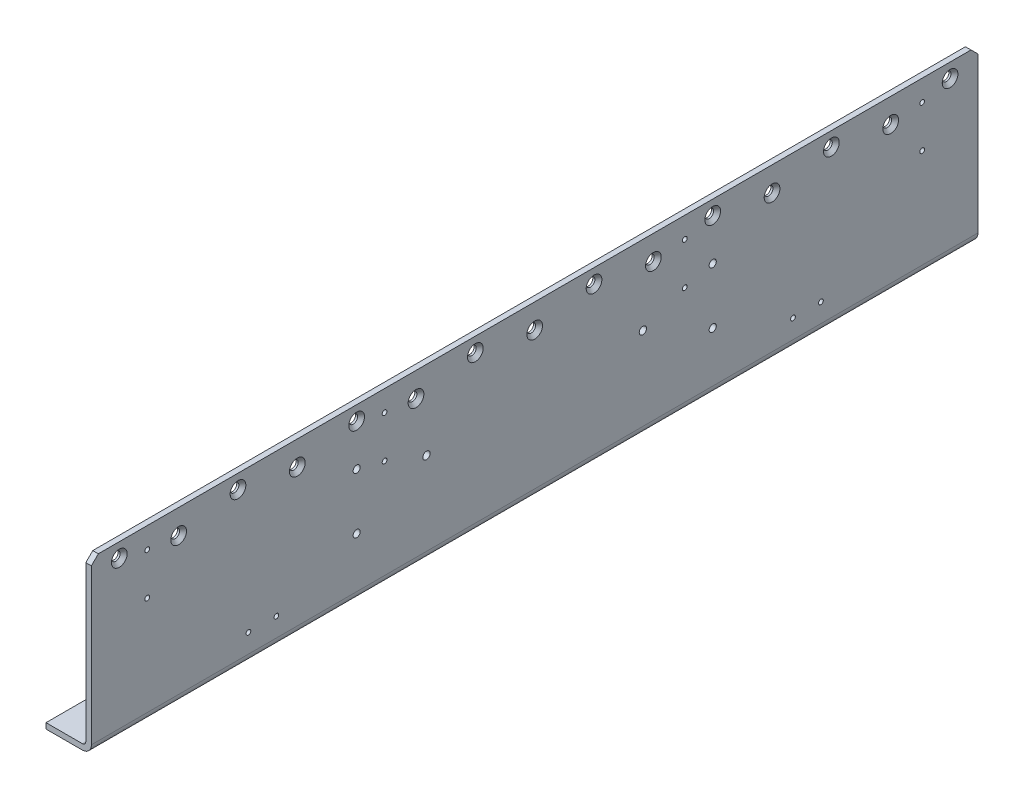
from build123d import *

# Parameters (mm, degrees)
BOSS_EXTRUDE1_DEPTH           = 1270
SKETCH3_R                     = 6.25
CUT_EXTRUDE1_DEPTH            = 3
SKETCH4_R                     = 6.25
CUT_EXTRUDE2_DEPTH            = 5
CUT_EXTRUDE2_DRAFT            = 45
CUT_EXTRUDE2_PROFILE_2_DEPTH  = 5
CUT_EXTRUDE2_PROFILE_2_DRAFT  = 45
CUT_EXTRUDE2_PROFILE_3_DEPTH  = 5
CUT_EXTRUDE2_PROFILE_3_DRAFT  = 45
CUT_EXTRUDE2_PROFILE_4_DEPTH  = 5
CUT_EXTRUDE2_PROFILE_4_DRAFT  = 45
CUT_EXTRUDE2_PROFILE_5_DEPTH  = 5
CUT_EXTRUDE2_PROFILE_5_DRAFT  = 45
CUT_EXTRUDE2_PROFILE_6_DEPTH  = 5
CUT_EXTRUDE2_PROFILE_6_DRAFT  = 45
CUT_EXTRUDE2_PROFILE_7_DEPTH  = 5
CUT_EXTRUDE2_PROFILE_7_DRAFT  = 45
CUT_EXTRUDE2_PROFILE_8_DEPTH  = 5
CUT_EXTRUDE2_PROFILE_8_DRAFT  = 45
CUT_EXTRUDE2_PROFILE_9_DEPTH  = 5
CUT_EXTRUDE2_PROFILE_9_DRAFT  = 45
CUT_EXTRUDE2_PROFILE_10_DEPTH = 5
CUT_EXTRUDE2_PROFILE_10_DRAFT = 45
CUT_EXTRUDE2_PROFILE_11_DEPTH = 5
CUT_EXTRUDE2_PROFILE_11_DRAFT = 45
CUT_EXTRUDE2_PROFILE_12_DEPTH = 5
CUT_EXTRUDE2_PROFILE_12_DRAFT = 45
CUT_EXTRUDE2_PROFILE_13_DEPTH = 5
CUT_EXTRUDE2_PROFILE_13_DRAFT = 45
CUT_EXTRUDE2_PROFILE_14_DEPTH = 5
CUT_EXTRUDE2_PROFILE_14_DRAFT = 45
CUT_EXTRUDE2_PROFILE_15_DEPTH = 5
CUT_EXTRUDE2_PROFILE_15_DRAFT = 45
SKETCH5_R                     = 3
SKETCH5_R_2                   = 5
SKETCH5_R_3                   = 5.25
CUT_EXTRUDE3_DEPTH            = 8
M12_TAPPED_HOLE1_D            = 10.2
M12_TAPPED_HOLE1_DEPTH        = 25.25
M12_TAPPED_HOLE1_TIP          = 3.064389157
M8_TAPPED_HOLE1_D             = 6.8
M8_TAPPED_HOLE1_DEPTH         = 19.75
M8_TAPPED_HOLE1_TIP           = 2.042926105
CHAMFER1_SIZE                 = 10
SKETCH10_R                    = 6.5
SKETCH10_R_2                  = 7.5
CUT_EXTRUDE4_DEPTH            = 8


with BuildPart() as part:
    # Sketch1 → Boss-Extrude1 (new body)
    with BuildSketch(Plane.XY):
        with BuildLine():
            Line((0, 0), (0, -232))
            ThreePointArc((0, -232), (-3.807611845, -241.192388155), (-13, -245))
            Line((-13, -245), (-65, -245))
            Line((-65, -245), (-65, -237))
            Line((-65, -237), (-13, -237))
            ThreePointArc((-13, -237), (-9.464466094, -235.535533906), (-8, -232))
            Line((-8, -232), (-8, 0))
            Line((-8, 0), (0, 0))
        make_face()
    extrude(amount=BOSS_EXTRUDE1_DEPTH)

    # Sketch3 → Cut-Extrude1 (cut)
    with BuildSketch(Plane.ZY.offset(8)):
        with Locations(Location((40, -20.5, 0), (0, 0, 270))):
            Circle(SKETCH3_R)
        with Locations(Location((210, -20.5, 0), (0, 0, 270))):
            Circle(SKETCH3_R)
        with Locations(Location((380, -20.5, 0), (0, 0, 270))):
            Circle(SKETCH3_R)
        with Locations(Location((550, -20.5, 0), (0, 0, 270))):
            Circle(SKETCH3_R)
        with Locations(Location((720, -20.5, 0), (0, 0, 270))):
            Circle(SKETCH3_R)
        with Locations(Location((890, -20.5, 0), (0, 0, 270))):
            Circle(SKETCH3_R)
        with Locations(Location((1060, -20.5, 0), (0, 0, 270))):
            Circle(SKETCH3_R)
        with Locations(Location((1230, -20.5, 0), (0, 0, 270))):
            Circle(SKETCH3_R)
        with Locations(Location((125, -35, 0), (0, 0, 270))):
            Circle(SKETCH3_R)
        with Locations(Location((295, -35, 0), (0, 0, 270))):
            Circle(SKETCH3_R)
        with Locations(Location((465, -35, 0), (0, 0, 270))):
            Circle(SKETCH3_R)
        with Locations(Location((635, -35, 0), (0, 0, 270))):
            Circle(SKETCH3_R)
        with Locations(Location((805, -35, 0), (0, 0, 270))):
            Circle(SKETCH3_R)
        with Locations(Location((975, -35, 0), (0, 0, 270))):
            Circle(SKETCH3_R)
        with Locations(Location((1145, -35, 0), (0, 0, 270))):
            Circle(SKETCH3_R)
    extrude(amount=-CUT_EXTRUDE1_DEPTH, mode=Mode.SUBTRACT)


with BuildPart() as cut_extrude2_tool:
    # Sketch4 → Cut-Extrude2 (with draft: the straight prism first)
    with BuildSketch(Plane.ZY.offset(5)):
        with Locations(Location((1230, -20.5, 0), (0, 0, 270))):
            Circle(SKETCH4_R)
    extrude(amount=-CUT_EXTRUDE2_DEPTH)
    # Cut-Extrude2: the draft: its side faces are tilted about the plane it starts from
    cut_extrude2_sides = [cut_extrude2_tool.faces().sort_by_distance(p)[0] for p in [
        (-2.5, -14.25, 1230),
    ]]
    draft(cut_extrude2_sides, Plane.ZY.offset(5), CUT_EXTRUDE2_DRAFT)


with BuildPart() as part_1:
    add(part.part)

    # Cut-Extrude2: cut by cut_extrude2_tool
    add(cut_extrude2_tool.part, mode=Mode.SUBTRACT)


with BuildPart() as cut_extrude2_profile_2_tool:
    # Sketch4 → Cut-Extrude2 profile 2 (with draft: the straight prism first)
    with BuildSketch(Plane.ZY.offset(5)):
        with Locations(Location((1145, -35, 0), (0, 0, 270))):
            Circle(SKETCH4_R)
    extrude(amount=-CUT_EXTRUDE2_PROFILE_2_DEPTH)
    # Cut-Extrude2 profile 2: the draft: its side faces are tilted about the plane it starts from
    cut_extrude2_profile_2_sides = [cut_extrude2_profile_2_tool.faces().sort_by_distance(p)[0] for p in [
        (-2.5, -28.75, 1145),
    ]]
    draft(cut_extrude2_profile_2_sides, Plane.ZY.offset(5), CUT_EXTRUDE2_PROFILE_2_DRAFT)


with BuildPart() as part_2:
    add(part_1.part)

    # Cut-Extrude2 profile 2: cut by cut_extrude2_profile_2_tool
    add(cut_extrude2_profile_2_tool.part, mode=Mode.SUBTRACT)


with BuildPart() as cut_extrude2_profile_3_tool:
    # Sketch4 → Cut-Extrude2 profile 3 (with draft: the straight prism first)
    with BuildSketch(Plane.ZY.offset(5)):
        with Locations(Location((1060, -20.5, 0), (0, 0, 270))):
            Circle(SKETCH4_R)
    extrude(amount=-CUT_EXTRUDE2_PROFILE_3_DEPTH)
    # Cut-Extrude2 profile 3: the draft: its side faces are tilted about the plane it starts from
    cut_extrude2_profile_3_sides = [cut_extrude2_profile_3_tool.faces().sort_by_distance(p)[0] for p in [
        (-2.5, -14.25, 1060),
    ]]
    draft(cut_extrude2_profile_3_sides, Plane.ZY.offset(5), CUT_EXTRUDE2_PROFILE_3_DRAFT)


with BuildPart() as part_3:
    add(part_2.part)

    # Cut-Extrude2 profile 3: cut by cut_extrude2_profile_3_tool
    add(cut_extrude2_profile_3_tool.part, mode=Mode.SUBTRACT)


with BuildPart() as cut_extrude2_profile_4_tool:
    # Sketch4 → Cut-Extrude2 profile 4 (with draft: the straight prism first)
    with BuildSketch(Plane.ZY.offset(5)):
        with Locations(Location((975, -35, 0), (0, 0, 270))):
            Circle(SKETCH4_R)
    extrude(amount=-CUT_EXTRUDE2_PROFILE_4_DEPTH)
    # Cut-Extrude2 profile 4: the draft: its side faces are tilted about the plane it starts from
    cut_extrude2_profile_4_sides = [cut_extrude2_profile_4_tool.faces().sort_by_distance(p)[0] for p in [
        (-2.5, -28.75, 975),
    ]]
    draft(cut_extrude2_profile_4_sides, Plane.ZY.offset(5), CUT_EXTRUDE2_PROFILE_4_DRAFT)


with BuildPart() as part_4:
    add(part_3.part)

    # Cut-Extrude2 profile 4: cut by cut_extrude2_profile_4_tool
    add(cut_extrude2_profile_4_tool.part, mode=Mode.SUBTRACT)


with BuildPart() as cut_extrude2_profile_5_tool:
    # Sketch4 → Cut-Extrude2 profile 5 (with draft: the straight prism first)
    with BuildSketch(Plane.ZY.offset(5)):
        with Locations(Location((890, -20.5, 0), (0, 0, 270))):
            Circle(SKETCH4_R)
    extrude(amount=-CUT_EXTRUDE2_PROFILE_5_DEPTH)
    # Cut-Extrude2 profile 5: the draft: its side faces are tilted about the plane it starts from
    cut_extrude2_profile_5_sides = [cut_extrude2_profile_5_tool.faces().sort_by_distance(p)[0] for p in [
        (-2.5, -14.25, 890),
    ]]
    draft(cut_extrude2_profile_5_sides, Plane.ZY.offset(5), CUT_EXTRUDE2_PROFILE_5_DRAFT)


with BuildPart() as part_5:
    add(part_4.part)

    # Cut-Extrude2 profile 5: cut by cut_extrude2_profile_5_tool
    add(cut_extrude2_profile_5_tool.part, mode=Mode.SUBTRACT)


with BuildPart() as cut_extrude2_profile_6_tool:
    # Sketch4 → Cut-Extrude2 profile 6 (with draft: the straight prism first)
    with BuildSketch(Plane.ZY.offset(5)):
        with Locations(Location((635, -35, 0), (0, 0, 270))):
            Circle(SKETCH4_R)
    extrude(amount=-CUT_EXTRUDE2_PROFILE_6_DEPTH)
    # Cut-Extrude2 profile 6: the draft: its side faces are tilted about the plane it starts from
    cut_extrude2_profile_6_sides = [cut_extrude2_profile_6_tool.faces().sort_by_distance(p)[0] for p in [
        (-2.5, -28.75, 635),
    ]]
    draft(cut_extrude2_profile_6_sides, Plane.ZY.offset(5), CUT_EXTRUDE2_PROFILE_6_DRAFT)


with BuildPart() as part_6:
    add(part_5.part)

    # Cut-Extrude2 profile 6: cut by cut_extrude2_profile_6_tool
    add(cut_extrude2_profile_6_tool.part, mode=Mode.SUBTRACT)


with BuildPart() as cut_extrude2_profile_7_tool:
    # Sketch4 → Cut-Extrude2 profile 7 (with draft: the straight prism first)
    with BuildSketch(Plane.ZY.offset(5)):
        with Locations(Location((550, -20.5, 0), (0, 0, 270))):
            Circle(SKETCH4_R)
    extrude(amount=-CUT_EXTRUDE2_PROFILE_7_DEPTH)
    # Cut-Extrude2 profile 7: the draft: its side faces are tilted about the plane it starts from
    cut_extrude2_profile_7_sides = [cut_extrude2_profile_7_tool.faces().sort_by_distance(p)[0] for p in [
        (-2.5, -14.25, 550),
    ]]
    draft(cut_extrude2_profile_7_sides, Plane.ZY.offset(5), CUT_EXTRUDE2_PROFILE_7_DRAFT)


with BuildPart() as part_7:
    add(part_6.part)

    # Cut-Extrude2 profile 7: cut by cut_extrude2_profile_7_tool
    add(cut_extrude2_profile_7_tool.part, mode=Mode.SUBTRACT)


with BuildPart() as cut_extrude2_profile_8_tool:
    # Sketch4 → Cut-Extrude2 profile 8 (with draft: the straight prism first)
    with BuildSketch(Plane.ZY.offset(5)):
        with Locations(Location((465, -35, 0), (0, 0, 270))):
            Circle(SKETCH4_R)
    extrude(amount=-CUT_EXTRUDE2_PROFILE_8_DEPTH)
    # Cut-Extrude2 profile 8: the draft: its side faces are tilted about the plane it starts from
    cut_extrude2_profile_8_sides = [cut_extrude2_profile_8_tool.faces().sort_by_distance(p)[0] for p in [
        (-2.5, -28.75, 465),
    ]]
    draft(cut_extrude2_profile_8_sides, Plane.ZY.offset(5), CUT_EXTRUDE2_PROFILE_8_DRAFT)


with BuildPart() as part_8:
    add(part_7.part)

    # Cut-Extrude2 profile 8: cut by cut_extrude2_profile_8_tool
    add(cut_extrude2_profile_8_tool.part, mode=Mode.SUBTRACT)


with BuildPart() as cut_extrude2_profile_9_tool:
    # Sketch4 → Cut-Extrude2 profile 9 (with draft: the straight prism first)
    with BuildSketch(Plane.ZY.offset(5)):
        with Locations(Location((380, -20.5, 0), (0, 0, 270))):
            Circle(SKETCH4_R)
    extrude(amount=-CUT_EXTRUDE2_PROFILE_9_DEPTH)
    # Cut-Extrude2 profile 9: the draft: its side faces are tilted about the plane it starts from
    cut_extrude2_profile_9_sides = [cut_extrude2_profile_9_tool.faces().sort_by_distance(p)[0] for p in [
        (-2.5, -14.25, 380),
    ]]
    draft(cut_extrude2_profile_9_sides, Plane.ZY.offset(5), CUT_EXTRUDE2_PROFILE_9_DRAFT)


with BuildPart() as part_9:
    add(part_8.part)

    # Cut-Extrude2 profile 9: cut by cut_extrude2_profile_9_tool
    add(cut_extrude2_profile_9_tool.part, mode=Mode.SUBTRACT)


with BuildPart() as cut_extrude2_profile_10_tool:
    # Sketch4 → Cut-Extrude2 profile 10 (with draft: the straight prism first)
    with BuildSketch(Plane.ZY.offset(5)):
        with Locations(Location((295, -35, 0), (0, 0, 270))):
            Circle(SKETCH4_R)
    extrude(amount=-CUT_EXTRUDE2_PROFILE_10_DEPTH)
    # Cut-Extrude2 profile 10: the draft: its side faces are tilted about the plane it starts from
    cut_extrude2_profile_10_sides = [cut_extrude2_profile_10_tool.faces().sort_by_distance(p)[0] for p in [
        (-2.5, -28.75, 295),
    ]]
    draft(cut_extrude2_profile_10_sides, Plane.ZY.offset(5), CUT_EXTRUDE2_PROFILE_10_DRAFT)


with BuildPart() as part_10:
    add(part_9.part)

    # Cut-Extrude2 profile 10: cut by cut_extrude2_profile_10_tool
    add(cut_extrude2_profile_10_tool.part, mode=Mode.SUBTRACT)


with BuildPart() as cut_extrude2_profile_11_tool:
    # Sketch4 → Cut-Extrude2 profile 11 (with draft: the straight prism first)
    with BuildSketch(Plane.ZY.offset(5)):
        with Locations(Location((210, -20.5, 0), (0, 0, 270))):
            Circle(SKETCH4_R)
    extrude(amount=-CUT_EXTRUDE2_PROFILE_11_DEPTH)
    # Cut-Extrude2 profile 11: the draft: its side faces are tilted about the plane it starts from
    cut_extrude2_profile_11_sides = [cut_extrude2_profile_11_tool.faces().sort_by_distance(p)[0] for p in [
        (-2.5, -14.25, 210),
    ]]
    draft(cut_extrude2_profile_11_sides, Plane.ZY.offset(5), CUT_EXTRUDE2_PROFILE_11_DRAFT)


with BuildPart() as part_11:
    add(part_10.part)

    # Cut-Extrude2 profile 11: cut by cut_extrude2_profile_11_tool
    add(cut_extrude2_profile_11_tool.part, mode=Mode.SUBTRACT)


with BuildPart() as cut_extrude2_profile_12_tool:
    # Sketch4 → Cut-Extrude2 profile 12 (with draft: the straight prism first)
    with BuildSketch(Plane.ZY.offset(5)):
        with Locations(Location((125, -35, 0), (0, 0, 270))):
            Circle(SKETCH4_R)
    extrude(amount=-CUT_EXTRUDE2_PROFILE_12_DEPTH)
    # Cut-Extrude2 profile 12: the draft: its side faces are tilted about the plane it starts from
    cut_extrude2_profile_12_sides = [cut_extrude2_profile_12_tool.faces().sort_by_distance(p)[0] for p in [
        (-2.5, -28.75, 125),
    ]]
    draft(cut_extrude2_profile_12_sides, Plane.ZY.offset(5), CUT_EXTRUDE2_PROFILE_12_DRAFT)


with BuildPart() as part_12:
    add(part_11.part)

    # Cut-Extrude2 profile 12: cut by cut_extrude2_profile_12_tool
    add(cut_extrude2_profile_12_tool.part, mode=Mode.SUBTRACT)


with BuildPart() as cut_extrude2_profile_13_tool:
    # Sketch4 → Cut-Extrude2 profile 13 (with draft: the straight prism first)
    with BuildSketch(Plane.ZY.offset(5)):
        with Locations(Location((40, -20.5, 0), (0, 0, 270))):
            Circle(SKETCH4_R)
    extrude(amount=-CUT_EXTRUDE2_PROFILE_13_DEPTH)
    # Cut-Extrude2 profile 13: the draft: its side faces are tilted about the plane it starts from
    cut_extrude2_profile_13_sides = [cut_extrude2_profile_13_tool.faces().sort_by_distance(p)[0] for p in [
        (-2.5, -14.25, 40),
    ]]
    draft(cut_extrude2_profile_13_sides, Plane.ZY.offset(5), CUT_EXTRUDE2_PROFILE_13_DRAFT)


with BuildPart() as part_13:
    add(part_12.part)

    # Cut-Extrude2 profile 13: cut by cut_extrude2_profile_13_tool
    add(cut_extrude2_profile_13_tool.part, mode=Mode.SUBTRACT)


with BuildPart() as cut_extrude2_profile_14_tool:
    # Sketch4 → Cut-Extrude2 profile 14 (with draft: the straight prism first)
    with BuildSketch(Plane.ZY.offset(5)):
        with Locations(Location((805, -35, 0), (0, 0, 270))):
            Circle(SKETCH4_R)
    extrude(amount=-CUT_EXTRUDE2_PROFILE_14_DEPTH)
    # Cut-Extrude2 profile 14: the draft: its side faces are tilted about the plane it starts from
    cut_extrude2_profile_14_sides = [cut_extrude2_profile_14_tool.faces().sort_by_distance(p)[0] for p in [
        (-2.5, -28.75, 805),
    ]]
    draft(cut_extrude2_profile_14_sides, Plane.ZY.offset(5), CUT_EXTRUDE2_PROFILE_14_DRAFT)


with BuildPart() as part_14:
    add(part_13.part)

    # Cut-Extrude2 profile 14: cut by cut_extrude2_profile_14_tool
    add(cut_extrude2_profile_14_tool.part, mode=Mode.SUBTRACT)


with BuildPart() as cut_extrude2_profile_15_tool:
    # Sketch4 → Cut-Extrude2 profile 15 (with draft: the straight prism first)
    with BuildSketch(Plane.ZY.offset(5)):
        with Locations(Location((720, -20.5, 0), (0, 0, 270))):
            Circle(SKETCH4_R)
    extrude(amount=-CUT_EXTRUDE2_PROFILE_15_DEPTH)
    # Cut-Extrude2 profile 15: the draft: its side faces are tilted about the plane it starts from
    cut_extrude2_profile_15_sides = [cut_extrude2_profile_15_tool.faces().sort_by_distance(p)[0] for p in [
        (-2.5, -14.25, 720),
    ]]
    draft(cut_extrude2_profile_15_sides, Plane.ZY.offset(5), CUT_EXTRUDE2_PROFILE_15_DRAFT)


with BuildPart() as part_15:
    add(part_14.part)

    # Cut-Extrude2 profile 15: cut by cut_extrude2_profile_15_tool
    add(cut_extrude2_profile_15_tool.part, mode=Mode.SUBTRACT)

    # Sketch5 → Cut-Extrude3 (cut)
    with BuildSketch(Plane(origin=(0, 0, 0), x_dir=(0, 0, -1), z_dir=(1, 0, 0))):
        with Locations(Location((-1190, -30, 0), (0, 0, 90))):
            Circle(SKETCH5_R)
        with Locations(Location((-1190, -90, 0), (0, 0, 90))):
            Circle(SKETCH5_R)
        with Locations(Location((-1045, -205, 0), (0, 0, 90))):
            Circle(SKETCH5_R)
        with Locations(Location((-1005, -205, 0), (0, 0, 90))):
            Circle(SKETCH5_R)
        with Locations(Location((-850, -30, 0), (0, 0, 90))):
            Circle(SKETCH5_R)
        with Locations(Location((-850, -90, 0), (0, 0, 90))):
            Circle(SKETCH5_R)
        with Locations(Location((-890, -80, 0), (0, 0, 90))):
            Circle(SKETCH5_R_2)
        with Locations(Location((-890, -160, 0), (0, 0, 90))):
            Circle(SKETCH5_R_2)
        with Locations(Location((-790, -113, 0), (0, 0, 90))):
            Circle(SKETCH5_R_3)
        with Locations(Location((-480, -113, 0), (0, 0, 270))):
            Circle(SKETCH5_R_3)
        with Locations(Location((-265, -205, 0), (0, 0, 270))):
            Circle(SKETCH5_R)
        with Locations(Location((-225, -205, 0), (0, 0, 270))):
            Circle(SKETCH5_R)
        with Locations(Location((-420, -30, 0), (0, 0, 270))):
            Circle(SKETCH5_R)
        with Locations(Location((-420, -90, 0), (0, 0, 270))):
            Circle(SKETCH5_R)
        with Locations(Location((-380, -80, 0), (0, 0, 270))):
            Circle(SKETCH5_R_2)
        with Locations(Location((-380, -160, 0), (0, 0, 270))):
            Circle(SKETCH5_R_2)
        with Locations(Location((-80, -90, 0), (0, 0, 270))):
            Circle(SKETCH5_R)
        with Locations(Location((-80, -30, 0), (0, 0, 270))):
            Circle(SKETCH5_R)
    extrude(amount=-CUT_EXTRUDE3_DEPTH, mode=Mode.SUBTRACT)

    # M12 Tapped Hole1
    with Locations(Plane(origin=(0, 0, 0), x_dir=(0, 0, -1), z_dir=(1, 0, 0))):
        with Locations((-890, -80), (-890, -160), (-380, -80), (-380, -160)):
            Hole(M12_TAPPED_HOLE1_D / 2, depth=M12_TAPPED_HOLE1_DEPTH)
            with Locations((0, 0, -(M12_TAPPED_HOLE1_DEPTH + M12_TAPPED_HOLE1_TIP / 2))):  # 118° drill point
                Cone(0, M12_TAPPED_HOLE1_D / 2, M12_TAPPED_HOLE1_TIP, mode=Mode.SUBTRACT)

    # M8 Tapped Hole1
    with Locations(Plane(origin=(0, 0, 0), x_dir=(0, 0, -1), z_dir=(1, 0, 0))):
        with Locations((-1190, -30), (-1190, -90), (-1045, -205), (-1005, -205), (-850, -90), (-850, -30), (-420, -90), (-420, -30), (-265, -205), (-225, -205), (-80, -90), (-80, -30)):
            Hole(M8_TAPPED_HOLE1_D / 2, depth=M8_TAPPED_HOLE1_DEPTH)
            with Locations((0, 0, -(M8_TAPPED_HOLE1_DEPTH + M8_TAPPED_HOLE1_TIP / 2))):  # 118° drill point
                Cone(0, M8_TAPPED_HOLE1_D / 2, M8_TAPPED_HOLE1_TIP, mode=Mode.SUBTRACT)

    # Chamfer1
    chamfer1_edges = [part_15.edges().sort_by_distance(p)[0] for p in [
        (-4, 0, 1270),
        (-4, 0, 0),
    ]]
    chamfer(chamfer1_edges, length=CHAMFER1_SIZE)

    # Sketch10 → Cut-Extrude4 (cut)
    with BuildSketch(Plane(origin=(0, -237, 0), x_dir=(1, 0, 0), z_dir=(0, 1, 0))):
        with Locations(Location((-40, -890, 0), (0, 0, 270))):
            Circle(SKETCH10_R)
        with Locations(Location((-40, -380, 0), (0, 0, 270))):
            Circle(SKETCH10_R)
        with Locations(Location((-40, -537.5, 0), (0, 0, 270))):
            Circle(SKETCH10_R)
        with Locations(Location((-40, -732.5, 0), (0, 0, 270))):
            Circle(SKETCH10_R)
        with Locations(Location((-40, -635, 0), (0, 0, 270))):
            Circle(SKETCH10_R_2)
    extrude(amount=-CUT_EXTRUDE4_DEPTH, mode=Mode.SUBTRACT)


solid = part_15.part
